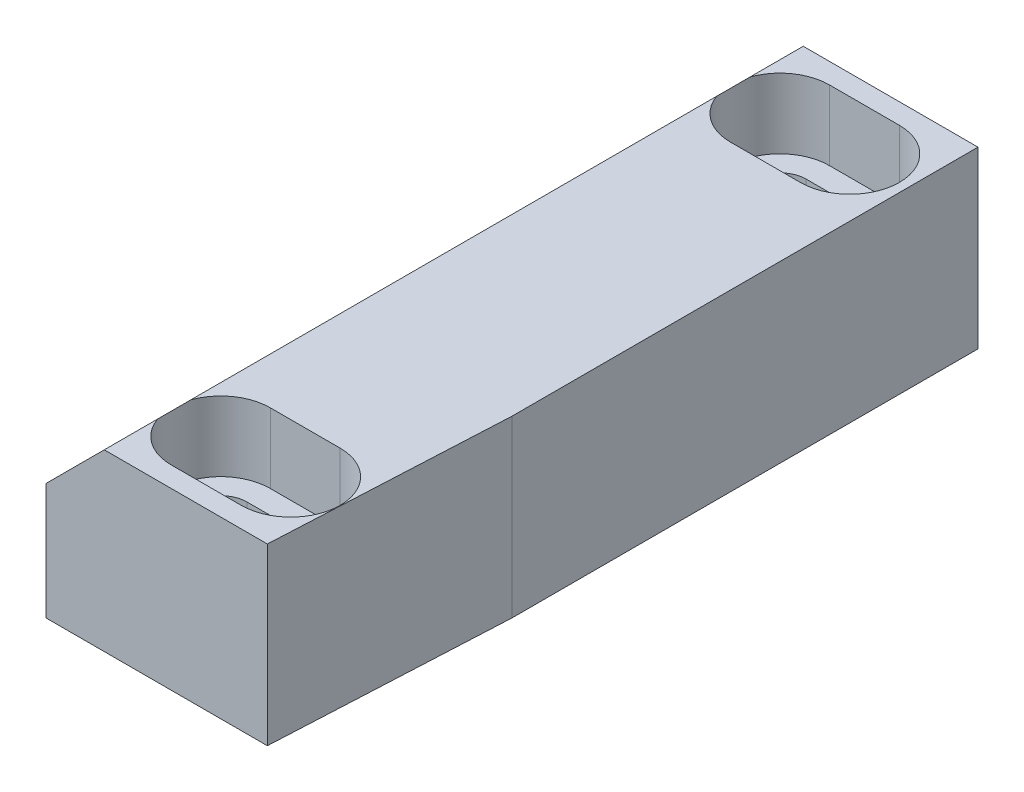
from build123d import *

# Parameters (mm, degrees)
SKETCH1_W           = 20
SKETCH1_H           = 60
BOSS_EXTRUDE1_DEPTH = 15
CHAMFER1_SIZE       = 5
CUT_EXTRUDE1_DEPTH  = 36
CUT_EXTRUDE2_DEPTH  = 36
CUT_EXTRUDE3_DEPTH  = 6


with BuildPart() as part:
    # Sketch1 → Boss-Extrude1 (new body)
    with BuildSketch(Plane(origin=(0, 0, 0), x_dir=(1, 0, 0), z_dir=(0, 1, 0))):
        Rectangle(SKETCH1_W, SKETCH1_H)
    extrude(amount=BOSS_EXTRUDE1_DEPTH)

    # Chamfer1
    chamfer1_edges = [part.edges().sort_by_distance(p)[0] for p in [
        (-10, 15, 0),
    ]]
    chamfer(chamfer1_edges, length=CHAMFER1_SIZE)

    # Sketch2 → Cut-Extrude1 (cut, through all)
    with BuildSketch(Plane(origin=(0, 15, 0), x_dir=(1, 0, 0), z_dir=(0, 1, 0))):
        Polygon((10, -30), (9, -30), (10, -10), align=None)
    extrude(amount=-CUT_EXTRUDE1_DEPTH, mode=Mode.SUBTRACT)

    # Sketch3 → Cut-Extrude2 (cut, through all)
    with BuildSketch(Plane(origin=(0, 15, 0), x_dir=(1, 0, 0), z_dir=(0, 1, 0))):
        with BuildLine():
            Line((5, 21.75), (-1, 21.75))
            ThreePointArc((-1, 21.75), (-3.25, 24), (-1, 26.25))
            Line((-1, 26.25), (5, 26.25))
            ThreePointArc((5, 26.25), (7.25, 24), (5, 21.75))
        make_face()
    cut_extrude2 = extrude(amount=-CUT_EXTRUDE2_DEPTH, mode=Mode.SUBTRACT)

    # Sketch4 → Cut-Extrude3 (cut)
    with BuildSketch(Plane(origin=(0, 15, 0), x_dir=(1, 0, 0), z_dir=(0, 1, 0))):
        with BuildLine():
            Line((-1, 19.75), (5, 19.75))
            ThreePointArc((5, 19.75), (9.25, 24), (5, 28.25))
            Line((5, 28.25), (-1, 28.25))
            ThreePointArc((-1, 28.25), (-5.25, 24), (-1, 19.75))
        make_face()
    cut_extrude3 = extrude(amount=-CUT_EXTRUDE3_DEPTH, mode=Mode.SUBTRACT)

    # Mirror1: Cut-Extrude2, Cut-Extrude3 across plane
    add(cut_extrude2.mirror(Plane.XY), mode=Mode.SUBTRACT)
    add(cut_extrude3.mirror(Plane.XY), mode=Mode.SUBTRACT)


solid = part.part
